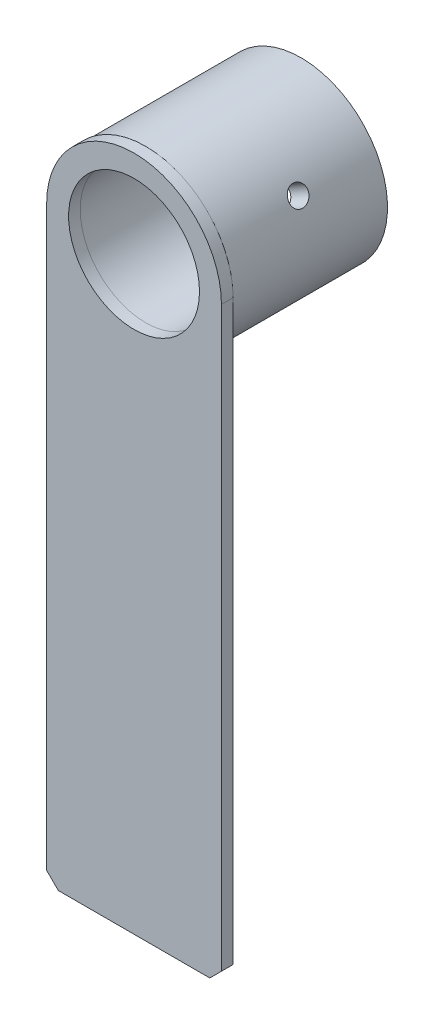
SolidWorks part; units mm, degrees
material "1023 碳钢板 (SS)"
ref_plane "前视基准面" through (0, 0, 0) normal (0, 0, 1) x (1, 0, 0)
ref_plane "上视基准面" through (0, 0, 0) normal (0, 1, 0) x (1, 0, 0)
ref_plane "右视基准面" through (0, 0, 0) normal (1, 0, 0) x (0, 0, -1)
ref_plane "基准面4" through (0, 0, 20) normal (0, 0, -1) x (-1, 0, 0)
sketch "草图1" plane through (0, 0, 20) normal (0, 0, -1) x (-1, 0, 0)
  line L0 (-22.5, 0) -> (-22.5, -151.6854)
  line L1 (-22.5, -151.6854) -> (22.5, -151.6854)
  line L2 (22.5, -151.6854) -> (22.5, 0)
  arc A0 (22.5, 0) -> (-22.5, 0) centre (0, 0) ccw
  dimension "D1" = 45
extrude "凸台-拉伸1" add sketch "草图1" against normal blind 3
sketch "草图2" plane through (0, 0, 20) normal (0, 0, -1) x (-1, 0, 0)
  circle A0 centre (0, 0) radius 22.25
extrude "凸台-拉伸2" add sketch "草图2" along normal blind 40 separate body
hole_wizard "M30 间隙孔1" positions "草图4" profile "草图3" hole size "M30" standard "ANSI Metric"
sketch "草图4" plane through (0, 0, 23) normal (0, 0, 1) x (1, 0, 0)
  point P0 (0, 0)
sketch "草图3" plane through (0, 0, 23) normal (1, 0, 0) x (0, -1, 0)
  line L0 (0, 0) -> (0, 43)
  line L1 (0, 43) -> (16.85, 43)
  line L2 (16.85, 43) -> (16.85, 0)
  line L5 (16.85, 0) -> (0, 0)
  line L11 (0, -6.35) -> (0, 107.95) construction
  dimension "通孔孔直径" = 33.7
  dimension "通孔孔深度" = 43
hole_wizard "Ø5.0 (5) 直径孔1" positions "3D草图1" profile "草图5" hole size "Ø5.0" standard "ANSI Metric"
sketch3d "3D草图1"
  point P0 (-19.4856, 11.25, 0)
sketch "草图5" plane through (-19.4856, 11.25, 0) normal (0, 0, 1) x (-0.5, -0.866, 0)
  line L0 (0, 0) -> (0, 22.5)
  line L1 (0, 22.5) -> (2.5, 22.5)
  line L2 (2.5, 22.5) -> (2.5, 0)
  line L5 (2.5, 0) -> (0, 0)
  line L11 (0, -6.35) -> (0, 107.95) construction
  dimension "通孔孔直径" = 5
  dimension "通孔孔深度" = 22.5
ref_plane "基准面5" through (14.431, 8.3318, 0) normal (-0.866, -0.5, 0) x (0, 0, 1)
hole_wizard "Ø5.0 (5) 直径孔2" positions "草图7" profile "草图6" hole size "Ø5.0" standard "ANSI Metric"
sketch "草图7" plane through (14.431, 8.3318, 0) normal (-0.866, -0.5, 0) x (0, 0, 1)
  point P0 (0, 0)
sketch "草图6" plane through (14.431, 8.3318, 0) normal (0, 0, 1) x (0.5, -0.866, 0)
  line L0 (0, 0) -> (0, 14.0721)
  line L1 (0, 14.0721) -> (2.5, 14.0721)
  line L2 (2.5, 14.0721) -> (2.5, 0)
  line L5 (2.5, 0) -> (0, 0)
  line L11 (0, -6.35) -> (0, 107.95) construction
  dimension "通孔孔直径" = 5
  dimension "通孔孔深度" = 14.0721
chamfer "倒角1" distance 3 angle 45 2 edges at (-22.5, -151.6854, 21.5) (22.5, -151.6854, 21.5)
